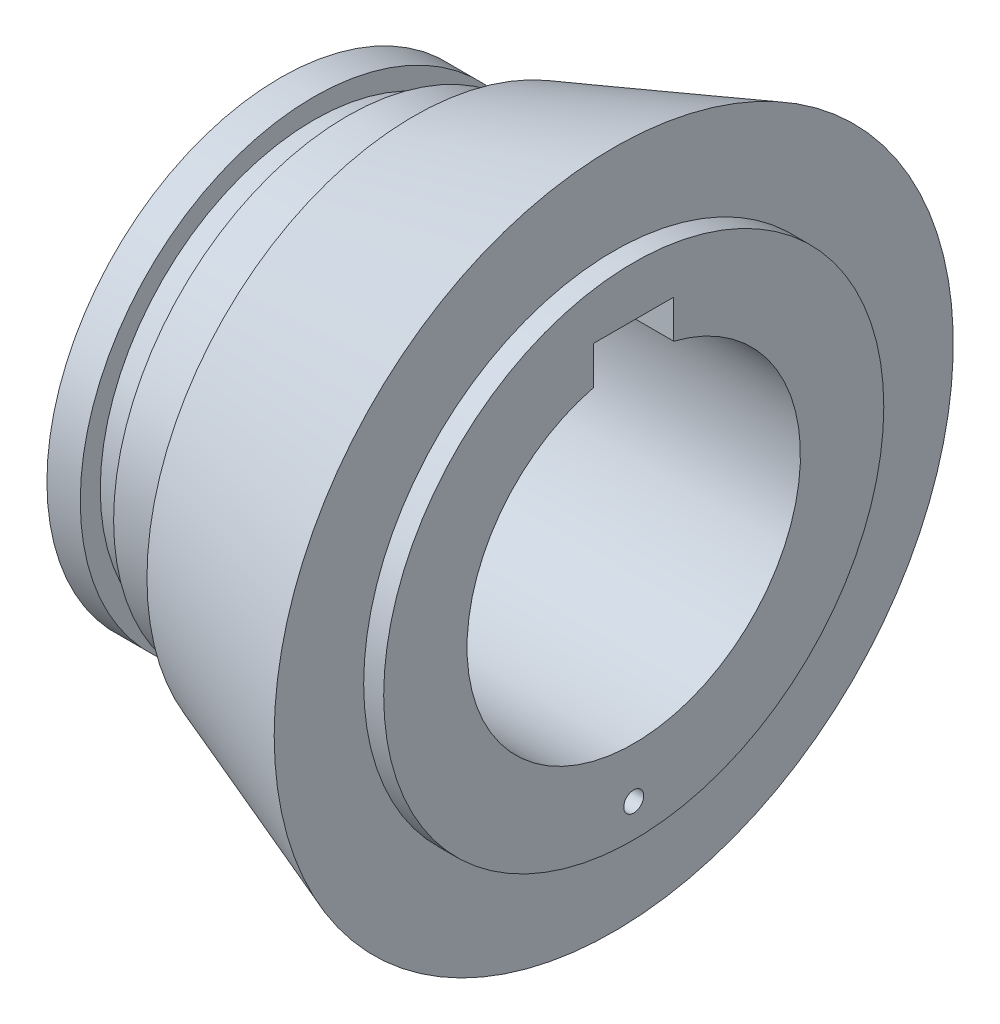
from build123d import *

# Parameters (mm, degrees)
SKETCH2_W          = 12
SKETCH2_H          = 12
CUT_EXTRUDE1_DEPTH = 90.412028951
SKETCH3_R          = 1.5
CUT_EXTRUDE2_DEPTH = 10


with BuildPart() as part:
    # Sketch1 → Revolve1 (revolve)
    with BuildSketch(Plane.XY, mode=Mode.PRIVATE) as revolve1_sk:
        Polygon((0, 25), (0, 35), (5, 35), (5, 32), (10, 32), (10, 35), (20, 35), (20, 40), (50, 50.919107028), (50, 37.5), (53, 37.5), (53, 25), align=None)
    revolve(revolve1_sk.sketch.rotate(Axis((0, 0, 0), (1, 0, 0)), 90), axis=Axis((0, 0, 0), (1, 0, 0)))

    # Sketch2 → Cut-Extrude1 (cut, through all)
    with BuildSketch(Plane(origin=(53, 0, 0), x_dir=(0, 0, -1), z_dir=(1, 0, 0))):
        with Locations((0, 24)):
            Rectangle(SKETCH2_W, SKETCH2_H)
    extrude(amount=-CUT_EXTRUDE1_DEPTH, mode=Mode.SUBTRACT)

    # Sketch3 → Cut-Extrude2 (cut)
    with BuildSketch(Plane(origin=(53, 0, 0), x_dir=(0, 0, -1), z_dir=(1, 0, 0))):
        with Locations((0, -32.5)):
            Circle(SKETCH3_R)
    extrude(amount=-CUT_EXTRUDE2_DEPTH, mode=Mode.SUBTRACT)


solid = part.part
